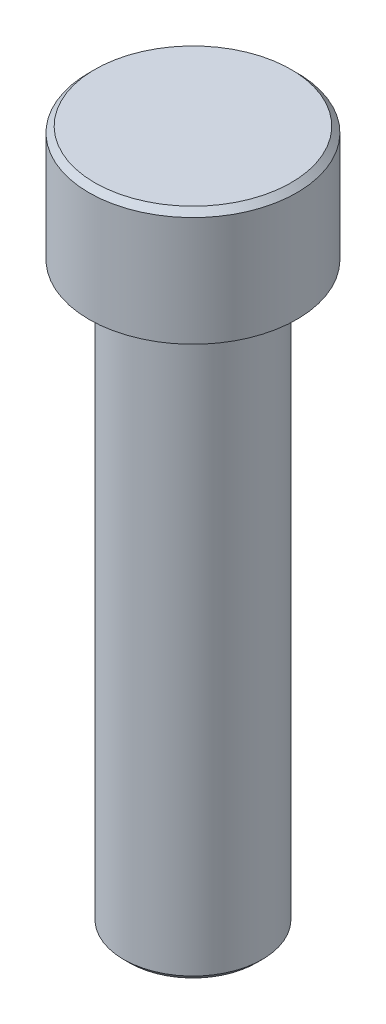
from build123d import *

# Parameters (mm, degrees)
SKETCH_1_R      = 6
EXTRUDE_1_DEPTH = 25
SKETCH_2_R      = 9
EXTRUDE_2_DEPTH = 10
CHAMFER_1_SIZE  = 0.5


with BuildPart() as part:
    # 草图1 → 凸台-拉伸1 (new, symmetric)
    with BuildSketch(Plane(origin=(0, 0, 0), x_dir=(1, 0, 0), z_dir=(0, 1, 0))):
        with Locations(Location((0, 0, 0), (0, 0, 270))):
            Circle(SKETCH_1_R)
    extrude(amount=EXTRUDE_1_DEPTH, both=True)

    # 草图2 → 凸台-拉伸2 (add)
    with BuildSketch(Plane(origin=(0, 25, 0), x_dir=(1, 0, 0), z_dir=(0, 1, 0))):
        with Locations(Location((0, 0, 0), (0, 0, 270))):
            Circle(SKETCH_2_R)
    extrude(amount=EXTRUDE_2_DEPTH)

    # 倒角1
    chamfer_1_edges = [part.edges().sort_by_distance(p)[0] for p in [
        (0, -25, -6),
        (0, 35, -9),
    ]]
    chamfer(chamfer_1_edges, length=CHAMFER_1_SIZE)


solid = part.part
